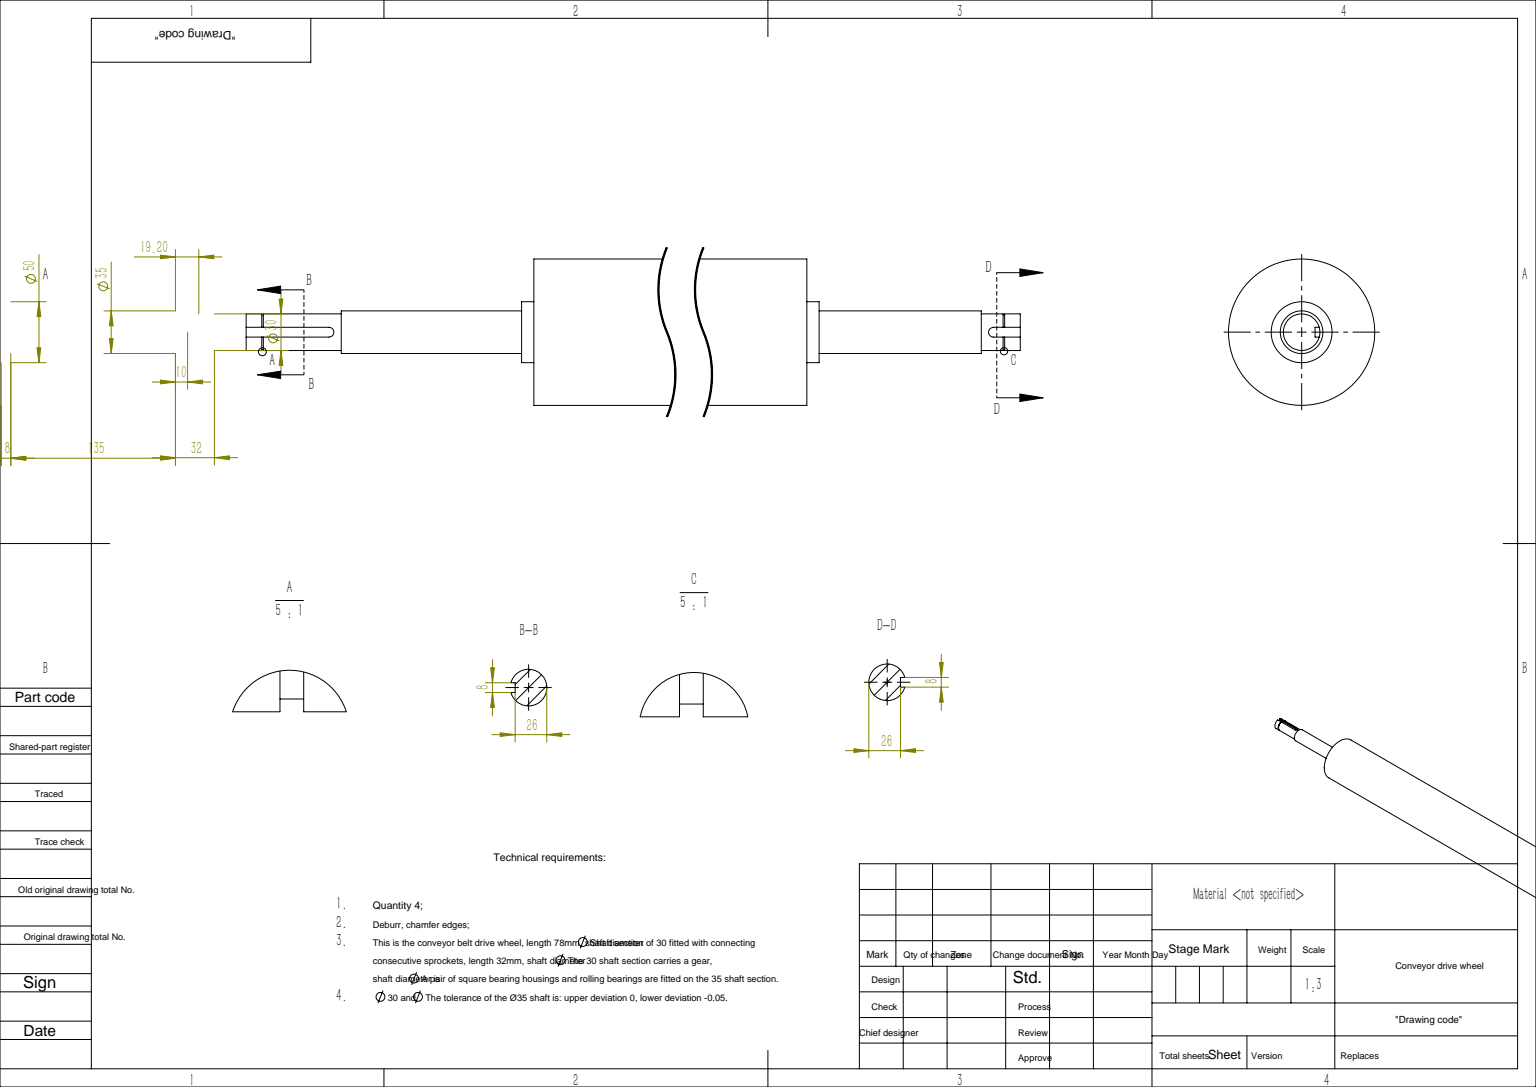
from build123d import *

# Parameters (mm, degrees)
CUT_EXTRUDE_1_DEPTH = 4
CUT_EXTRUDE_START   = -1.3
SKETCH_3_R          = 15
SKETCH_3_R_2        = 14.3
CUT_EXTRUDE_2_DEPTH = 1.3
CUT_EXTRUDE_3_DEPTH = 4
SKETCH_5_R          = 15
SKETCH_5_R_2        = 14.3
CUT_EXTRUDE_4_DEPTH = 1.3


with BuildPart() as part:
    # 草图1 → 旋转1 (revolve)
    with BuildSketch(Plane.XY, mode=Mode.PRIVATE) as revolve_1_sk:
        Polygon((0, 0), (0, 15), (78, 15), (78, 17.5), (226, 17.5), (226, 25), (236, 25), (236, 60), (1086, 60), (1086, 25), (1096, 25), (1096, 17.5), (1229, 17.5), (1229, 15), (1261, 15), (1261, 0), align=None)
    revolve(revolve_1_sk.sketch.rotate(Axis((0, 0, 0), (1, 0, 0)), 90), axis=Axis((0, 0, 0), (1, 0, 0)))

    # 草图2 → 切除-拉伸1 (cut)
    with BuildSketch(Plane(origin=(0, 15, 0), x_dir=(1, 0, 0), z_dir=(0, 1, 0))):
        with BuildLine():
            Line((68, 4), (-10, 4))
            Line((-10, 4), (-10, -4))
            Line((-10, -4), (68, -4))
            ThreePointArc((68, -4), (72, 0), (68, 4))
        make_face()
    extrude(amount=-CUT_EXTRUDE_1_DEPTH, mode=Mode.SUBTRACT)

    # 草图3 → 切除-拉伸2 (cut)
    with BuildSketch(Plane.ZY.offset(-12.8).offset(CUT_EXTRUDE_START)):
        Circle(SKETCH_3_R)
        Circle(SKETCH_3_R_2, mode=Mode.SUBTRACT)
    extrude(amount=CUT_EXTRUDE_2_DEPTH, mode=Mode.SUBTRACT)

    # 草图4 → 切除-拉伸3 (cut)
    with BuildSketch(Plane(origin=(0, 15, 0), x_dir=(1, 0, 0), z_dir=(0, 1, 0))):
        with BuildLine():
            Line((1239, 4), (1271, 4))
            Line((1271, 4), (1271, -4))
            Line((1271, -4), (1239, -4))
            ThreePointArc((1239, -4), (1235, 0), (1239, 4))
        make_face()
    extrude(amount=-CUT_EXTRUDE_3_DEPTH, mode=Mode.SUBTRACT)

    # 草图5 → 切除-拉伸4 (cut)
    with BuildSketch(Plane(origin=(1248.2, 0, 0), x_dir=(0, 0, -1), z_dir=(1, 0, 0))):
        with Locations(Location((0, 0, 0), (0, 0, 180))):
            Circle(SKETCH_5_R)
        Circle(SKETCH_5_R_2, mode=Mode.SUBTRACT)
    extrude(amount=-CUT_EXTRUDE_4_DEPTH, mode=Mode.SUBTRACT)


solid = part.part
